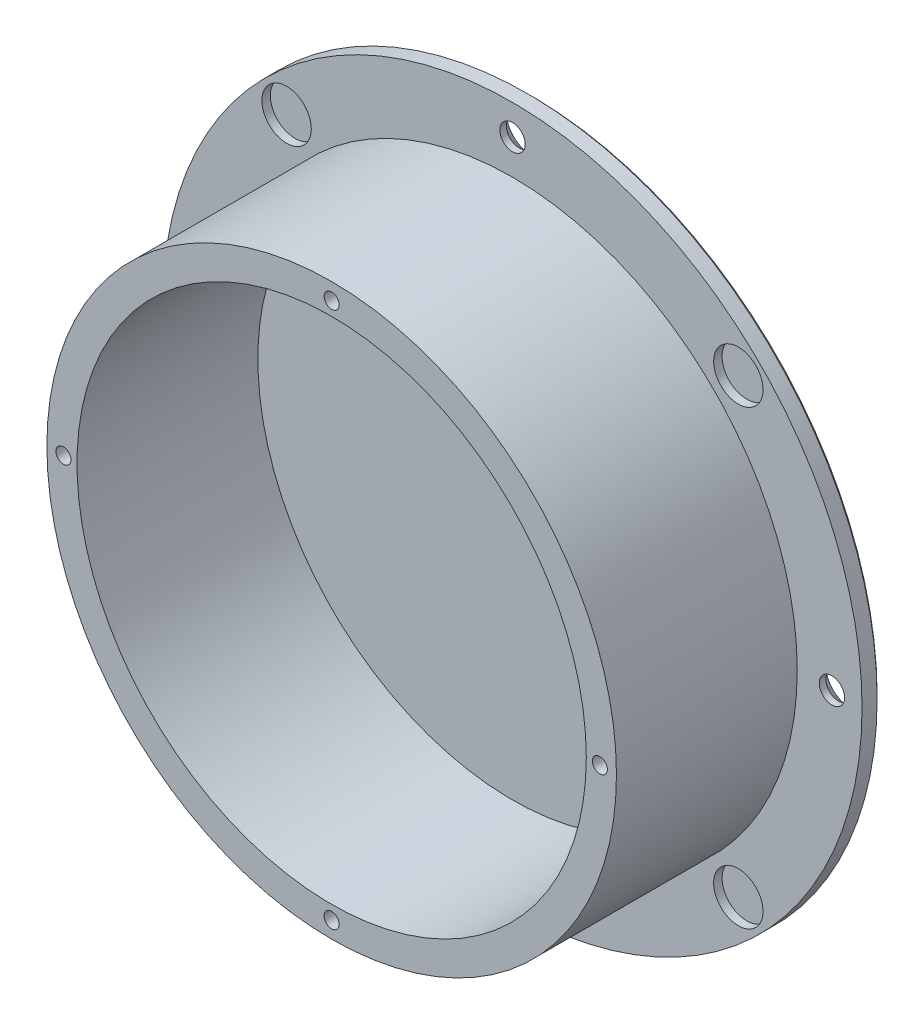
from build123d import *

# Parameters (mm, degrees)
SKETCH_1_R                   = 58
EXTRUDE_1_DEPTH              = 3
SKETCH_2_R                   = 47.25
SKETCH_2_R_2                 = 42.25
EXTRUDE_2_DEPTH              = 30
CHAMFER_1_SIZE               = 0.5
HOLE_WIZARD_M4_1_D           = 4.2
HOLE_WIZARD_M4_1_DEPTH       = 10.1
HOLE_WIZARD_M4_1_CSINK_D     = 8
HOLE_WIZARD_M4_1_CSINK_ANGLE = 90
HOLE_WIZARD_M4_1_TIP         = 1.2618073
HOLE_WIZARD_M3_2_D           = 2.5
HOLE_WIZARD_M3_2_DEPTH       = 7.5
HOLE_WIZARD_M3_2_TIP         = 0.751075774
SKETCH_32_R                  = 4.1
CUT_EXTRUDE_12_DEPTH         = 1.4


with BuildPart() as part:
    # 草图1 → 凸台-拉伸1 (new body)
    with BuildSketch(Plane.XY):
        Circle(SKETCH_1_R)
    extrude(amount=EXTRUDE_1_DEPTH)

    # 草图2 → 凸台-拉伸2 (add)
    with BuildSketch(Plane.XY.offset(3)):
        Circle(SKETCH_2_R)
        Circle(SKETCH_2_R_2, mode=Mode.SUBTRACT)
    extrude(amount=EXTRUDE_2_DEPTH)

    # 倒角1
    chamfer_1_edges = [part.edges().sort_by_distance(p)[0] for p in [
        (-58, 0, 0),
    ]]
    chamfer(chamfer_1_edges, length=CHAMFER_1_SIZE)

    # M4 六角凹锥坑螺钉的锥形沉头孔1
    with Locations(Plane(origin=(0, 0, 0), x_dir=(-1, 0, 0), z_dir=(0, 0, -1))):
        with Locations((0, 53), (53, 0), (0, -53), (-53, 0)):
            CounterSinkHole(HOLE_WIZARD_M4_1_D / 2, HOLE_WIZARD_M4_1_CSINK_D / 2, depth=HOLE_WIZARD_M4_1_DEPTH, counter_sink_angle=HOLE_WIZARD_M4_1_CSINK_ANGLE)
            with Locations((0, 0, -(HOLE_WIZARD_M4_1_DEPTH + HOLE_WIZARD_M4_1_TIP / 2))):  # 118° drill point
                Cone(0, HOLE_WIZARD_M4_1_D / 2, HOLE_WIZARD_M4_1_TIP, mode=Mode.SUBTRACT)

    # M3 螺纹孔2
    with Locations(Plane.XY.offset(33)):
        with Locations((0, 44.5), (44.5, 0), (0, -44.5), (-44.5, 0), (0, 0)):
            Hole(HOLE_WIZARD_M3_2_D / 2, depth=HOLE_WIZARD_M3_2_DEPTH)
            with Locations((0, 0, -(HOLE_WIZARD_M3_2_DEPTH + HOLE_WIZARD_M3_2_TIP / 2))):  # 118° drill point
                Cone(0, HOLE_WIZARD_M3_2_D / 2, HOLE_WIZARD_M3_2_TIP, mode=Mode.SUBTRACT)

    # 草图32 → 切除-拉伸12 (cut)
    with BuildSketch(Plane.XY.offset(3)):
        with Locations((37.476659403, -37.476659403)):
            Circle(SKETCH_32_R)
        with Locations(Location((37.476659403, 37.476659403, 0), (0, 0, 180))):
            Circle(SKETCH_32_R)
        with Locations((-37.476659403, 37.476659403)):
            Circle(SKETCH_32_R)
        with Locations(Location((-37.476659403, -37.476659403, 0), (0, 0, 180))):
            Circle(SKETCH_32_R)
    extrude(amount=-CUT_EXTRUDE_12_DEPTH, mode=Mode.SUBTRACT)


solid = part.part
